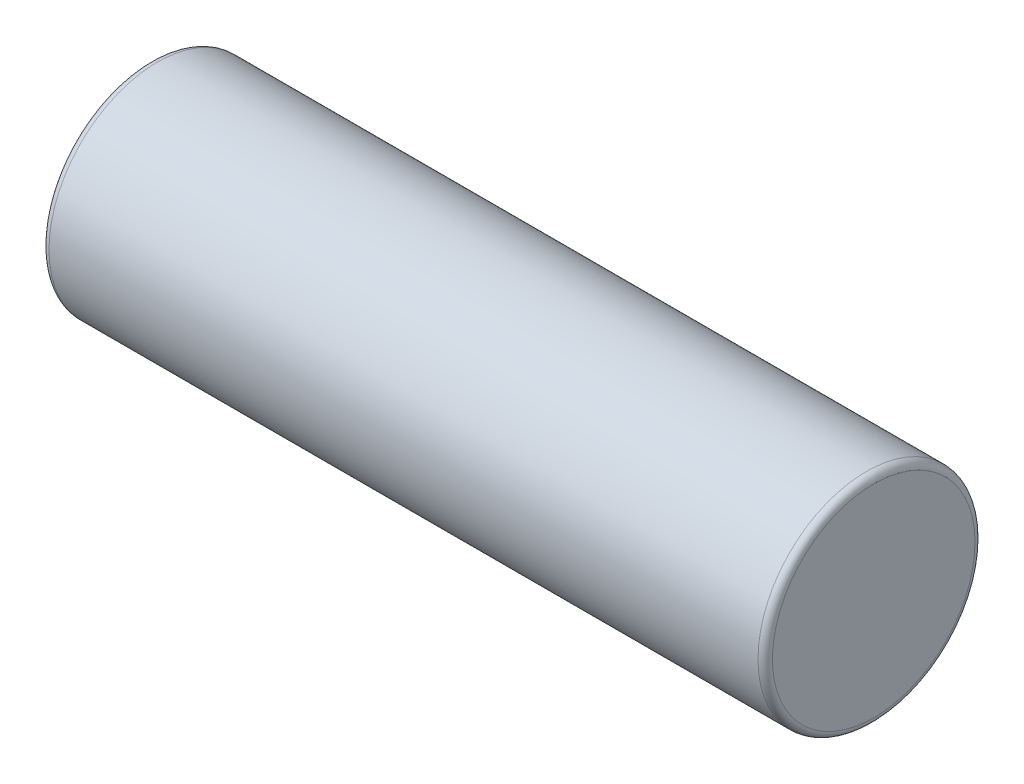
SolidWorks part; units mm, degrees
ref_plane "Front Plane" through (0, 0, 0) normal (0, 0, 1) x (1, 0, 0)
ref_plane "Top Plane" through (0, 0, 0) normal (0, 1, 0) x (1, 0, 0)
ref_plane "Right Plane" through (0, 0, 0) normal (1, 0, 0) x (0, 0, -1)
other "Configuration Table"
sketch "Sketch1" plane through (0, 0, 0) normal (1, 0, 0) x (0, 0, -1)
  circle A0 centre (0, 0) radius 30
  dimension "D1" = 60
extrude "Boss-Extrude1" add sketch "Sketch1" along normal blind 200
fillet "Fillet1" radius 2 2 edges at (0, 0, -30) (200, 0, -30)
